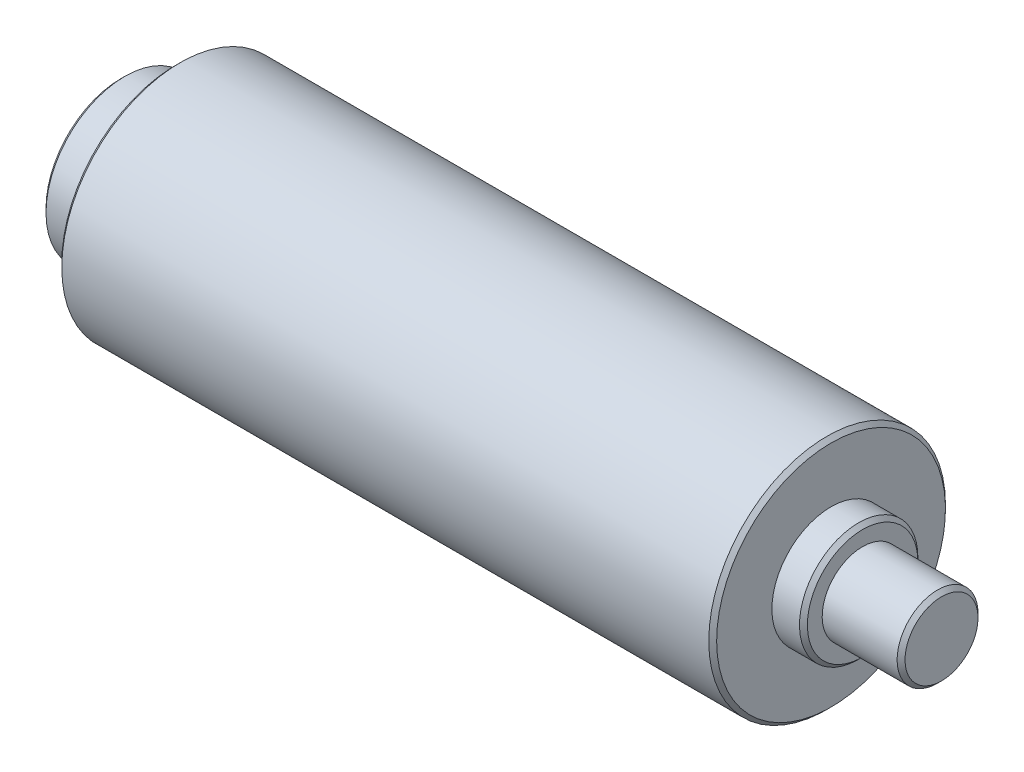
SolidWorks part; units mm, degrees
material "Q235B"
ref_plane "Front Plane" through (0, 0, 0) normal (0, 0, 1) x (1, 0, 0)
ref_plane "Top Plane" through (0, 0, 0) normal (0, 1, 0) x (1, 0, 0)
ref_plane "Right Plane" through (0, 0, 0) normal (1, 0, 0) x (0, 0, -1)
sketch "Sketch1" plane through (0, 0, 0) normal (0, 0, 1) x (1, 0, 0)
  line L0 (695.5088, 32.4746) -> (685.5088, 32.4746)
  line L1 (690.5088, 32.4746) -> (700.5088, 32.4746) construction
  line L2 (685.5088, 32.4746) -> (685.5088, 34.8496)
  line L3 (682.5088, 34.8496) -> (690.5088, 34.8496) construction
  line L4 (685.5088, 34.8496) -> (681.5088, 34.8496)
  line L5 (681.5088, 34.8496) -> (681.5088, 42.3496)
  line L6 (681.5088, 42.3496) -> (598.5088, 42.3496)
  line L7 (598.5088, -275) -> (598.5088, 225) construction
  line L8 (700.5088, 27.3496) -> (682.5088, 27.3496) construction
  line L9 (700.5088, 21.8648) -> (700.5088, 32.8344) construction
  line L10 (682.5088, -155.2055) -> (682.5088, 155.8496) construction
  line L11 (695.5088, 32.4746) -> (695.5088, 27.3496)
  line L12 (690.5088, -155.2055) -> (690.5088, 155.8496) construction
  line L13 (598.5088, 42.3496) -> (598.5088, 37.3496)
  line L14 (598.5088, 37.3496) -> (591.5088, 37.3496)
  line L15 (591.5088, 37.3496) -> (591.5088, 27.3496)
  line L16 (682.5088, 27.3496) -> (590.5088, 27.3496) construction
  line L17 (590.5088, -275) -> (590.5088, 225) construction
  line L18 (695.5088, 27.3496) -> (591.5088, 27.3496)
  dimension "D1" = 1
  dimension "D2" = 4
  dimension "D3" = 5
  dimension "D4" = 30
  dimension "D5" = 20
  dimension "D6" = 7
revolve "Revolve1" add sketch "Sketch1" angle 360 about L18
chamfer "Chamfer1" distance 0.5 angle 45 5 edges at (591.5088, 37.3496, 0) (598.5088, 42.3496, 0) (681.5088, 42.3496, 0) (685.5088, 34.8496, 0) (695.5088, 32.4746, 0)
